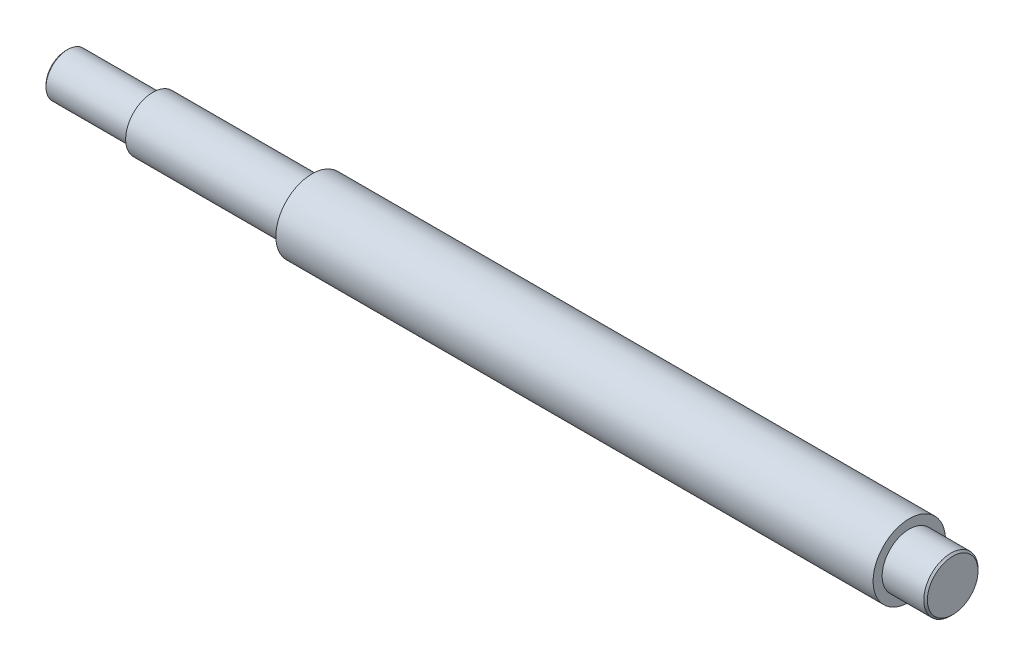
from build123d import *

# Parameters (mm, degrees)
CUT_EXTRUDE_1_DEPTH = 2.2
CHAMFER_1_SIZE      = 0.5


with BuildPart() as part:
    # 草图1 → 旋转1 (revolve)
    with BuildSketch(Plane(origin=(0, 0, 0), x_dir=(1, 0, 0), z_dir=(0, 1, 0)), mode=Mode.PRIVATE) as revolve_1_sk:
        Polygon((0, 0), (0, 6), (24, 6), (24, 7.5), (68, 7.5), (68, 10), (233, 10), (233, 7.5), (245, 7.5), (245, 0), align=None)
    revolve(revolve_1_sk.sketch.rotate(Axis((0, 0, 0), (1, 0, 0)), 180), axis=Axis((0, 0, 0), (1, 0, 0)))

    # 草图2 → 切除-拉伸1 (cut)
    with BuildSketch(Plane(origin=(0, -6, 0), x_dir=(-1, 0, 0), z_dir=(0, -1, 0))):
        with BuildLine():
            Line((-21, 2), (-3, 2))
            ThreePointArc((-3, 2), (-1, 0), (-3, -2))
            Line((-3, -2), (-21, -2))
            ThreePointArc((-21, -2), (-23, 0), (-21, 2))
        make_face()
    extrude(amount=-CUT_EXTRUDE_1_DEPTH, mode=Mode.SUBTRACT)

    # 倒角1
    chamfer_1_edges = [part.edges().sort_by_distance(p)[0] for p in [
        (0, 0, -6),
        (245, 0, -7.5),
    ]]
    chamfer(chamfer_1_edges, length=CHAMFER_1_SIZE)


solid = part.part
